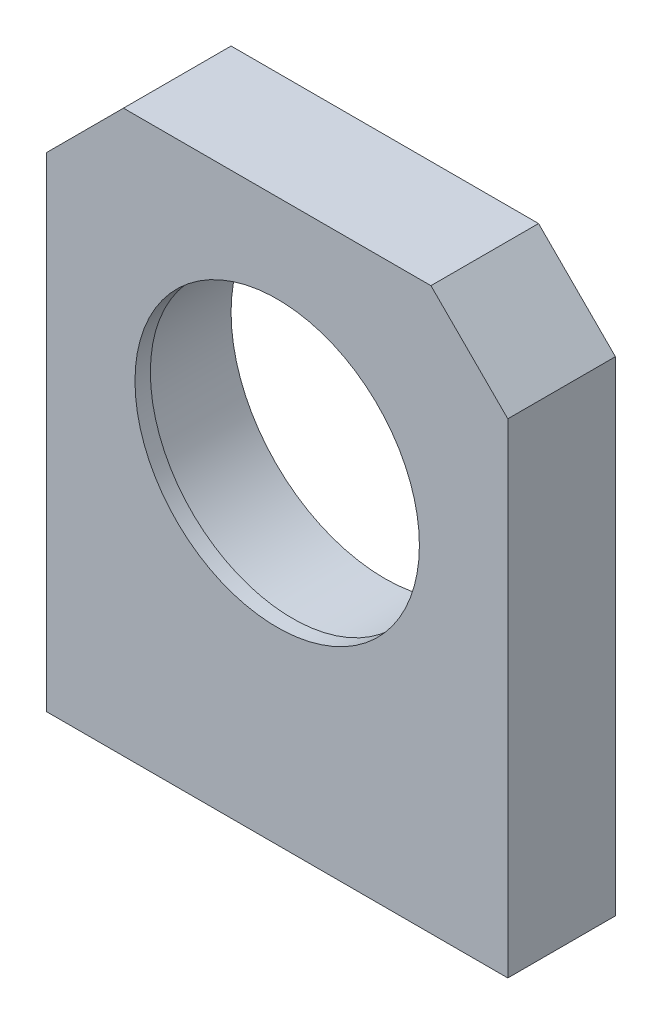
SolidWorks part; units mm, degrees
material "Q235A"
ref_plane "前视基准面" through (0, 0, 0) normal (0, 0, 1) x (1, 0, 0)
ref_plane "上视基准面" through (0, 0, 0) normal (0, 1, 0) x (1, 0, 0)
ref_plane "右视基准面" through (0, 0, 0) normal (1, 0, 0) x (0, 0, -1)
sketch "草图1" plane through (0, 0, 0) normal (0, 0, 1) x (1, 0, 0)
  line L1 (-30, -36.5) -> (30, -36.5)
  line L2 (-30, -36.5) -> (-30, 36.5)
  line L3 (-30, 36.5) -> (30, 36.5)
  line L4 (30, -36.5) -> (30, 36.5)
  line L5 (-30, -36.5) -> (30, 36.5) construction
  line L6 (-30, 36.5) -> (30, -36.5) construction
  circle A0 centre (0, 6.5) radius 20
  point P0 (0, 0)
  dimension "D1" = 40
  dimension "D2" = 30
  dimension "D3" = 43
  dimension "D4" = 60
extrude "凸台-拉伸1" add sketch "草图1" along normal mid plane 14
sketch "草图2" plane through (0, 0, 7) normal (0, 0, 1) x (1, 0, 0)
  circle A0 centre (0, 6.5) radius 20 construction
  circle A1 centre (0, 6.5) radius 20
  circle A2 centre (0, 6.5) radius 18.5
  dimension "D1" = 37
extrude "凸台-拉伸2" add sketch "草图2" against normal blind 2
chamfer "倒角1" distance 10 angle 45 2 edges at (30, 36.5, 0) (-30, 36.5, 0)
hole_wizard "M6 螺纹孔1" positions "3D草图1" profile "草图3" tap size "M6" standard "GB"
sketch3d "3D草图1"
  line L0 (-30, -36.5, 0) -> (30, -36.5, 0)
  line L1 (-30, -36.5, 7) -> (-30, -36.5, -7) construction
  line L2 (30, -36.5, 7) -> (30, -36.5, -7) construction
  point P0 (-24, -36.5, 0)
  point P2 (24, -36.5, 0)
sketch "草图3" plane through (-24, -36.5, 0) normal (1, 0, 0) x (0, 0, -1)
  line L0 (0, 0) -> (0, 15.5022)
  line L1 (0, 15.5022) -> (2.5, 14)
  line L2 (2.5, 14) -> (2.5, 0)
  line L5 (2.5, 0) -> (0, 0)
  line L10 (0, 15.5022) -> (-2.5, 14) construction
  line L11 (0, -6.35) -> (0, 107.95) construction
  dimension "螺纹孔钻头直径" = 5
  dimension "螺纹孔钻头深度" = 14
  dimension "导头角度" = 118
cosmetic thread "孔螺蚊线1"
cosmetic thread "孔螺蚊线2"
equation "\"D2@3D草图1\"=\"D1@3D草图1\""
